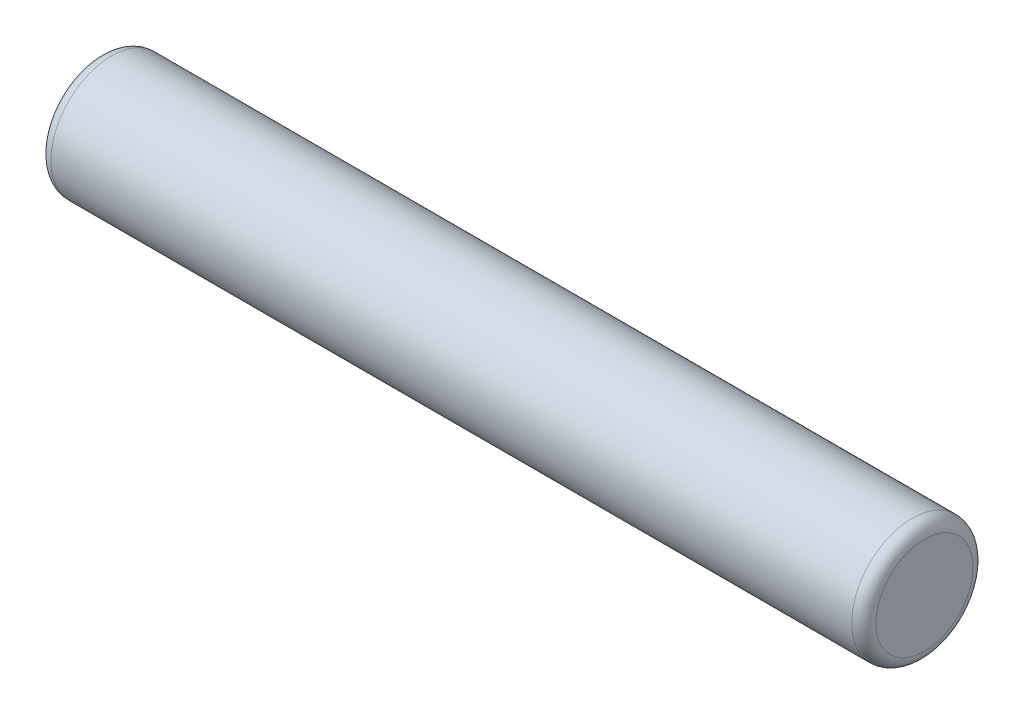
from build123d import *

# Parameters (mm, degrees)
SKETCH_1_R      = 1
EXTRUDE_1_DEPTH = 6.8
FILLET_1_R      = 0.2


with BuildPart() as part:
    # 草图1 → 凸台-拉伸1 (new, symmetric)
    with BuildSketch(Plane(origin=(0, 0, 0), x_dir=(0, 0, -1), z_dir=(1, 0, 0))):
        Circle(SKETCH_1_R)
    extrude(amount=EXTRUDE_1_DEPTH, both=True)

    # 圆角1
    fillet_1_edges = [part.edges().sort_by_distance(p)[0] for p in [
        (-6.8, 0, 1),
        (6.8, 0, 1),
    ]]
    fillet(fillet_1_edges, radius=FILLET_1_R)


solid = part.part
